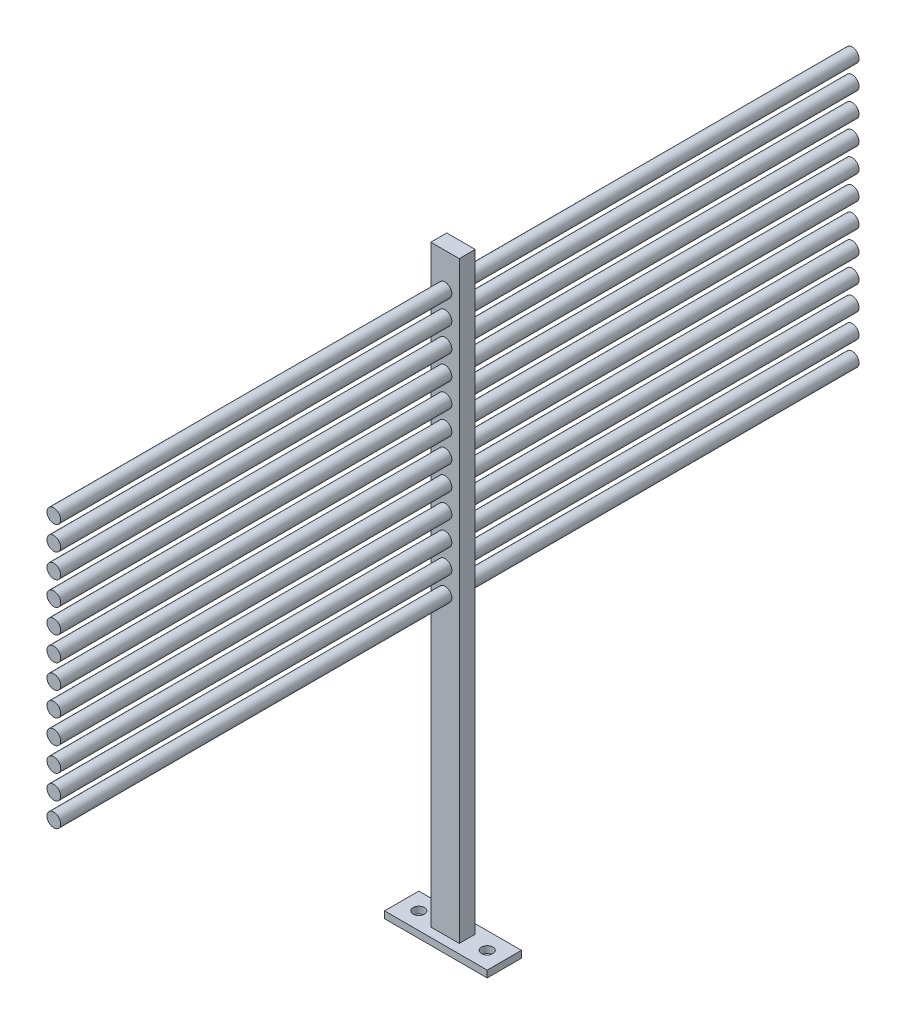
SolidWorks part; units mm, degrees
material "Q235"
ref_plane "Front Plane" through (0, 0, 0) normal (0, 0, 1) x (1, 0, 0)
ref_plane "Top Plane" through (0, 0, 0) normal (0, 1, 0) x (1, 0, 0)
ref_plane "Right Plane" through (0, 0, 0) normal (1, 0, 0) x (0, 0, -1)
sketch "Sketch1" plane through (0, 0, 0) normal (0, 0, 1) x (1, 0, 0)
  line L1 (-12.5, 260) -> (12.5, 260)
  line L2 (-12.5, 260) -> (-12.5, -260)
  line L3 (-12.5, -260) -> (12.5, -260)
  line L4 (12.5, 260) -> (12.5, -260)
  line L5 (-12.5, 260) -> (12.5, -260) construction
  line L6 (-12.5, -260) -> (12.5, 260) construction
  point P0 (0, 0)
  dimension "D1" = 25
  dimension "D2" = 520
extrude "Boss-Extrude1" add sketch "Sketch1" along normal blind 14
sketch "Sketch3" plane through (0, 0, 14) normal (0, 0, 1) x (1, 0, 0)
  line L0 (12.5, 260) -> (-12.5, 260) construction
  line L1 (12.5, -260) -> (12.5, 260) construction
  circle A0 centre (0, 230) radius 6
  dimension "D1" = 12
  dimension "D2" = 30
  dimension "D3" = 12.5
extrude "Boss-Extrude2" add sketch "Sketch3" along normal mid plane 700 from offset 7 offset against normal yes
pattern_linear "LPattern1" count 12 spacing 21 along (0, -1, 0) of "Boss-Extrude2"
sketch "Sketch4" plane through (0, -260, 0) normal (0, -1, 0) x (1, 0, 0)
  line L0 (-12.5, 14) -> (12.5, 0) construction
  line L2 (-45, 22) -> (45, 22)
  line L3 (-45, 22) -> (-45, -8)
  line L4 (-45, -8) -> (45, -8)
  line L5 (45, 22) -> (45, -8)
  line L6 (-45, 22) -> (45, -8) construction
  line L7 (-45, -8) -> (45, 22) construction
  point P4 (0, 7)
  dimension "D1" = 90
  dimension "D2" = 30
extrude "Boss-Extrude3" add sketch "Sketch4" along normal blind 6
sketch "Sketch5" plane through (0, 260, 0) normal (0, 1, 0) x (1, 0, 0)
  line L4 (-45, -22) -> (45, -22)
  line L5 (45, -22) -> (45, 8)
  line L6 (45, 8) -> (-45, 8)
  line L7 (-45, 8) -> (-45, -22)
  line L8 (-45, -22) -> (45, -22)
  line L9 (45, -22) -> (45, 8)
  line L10 (45, 8) -> (-45, 8)
  line L11 (-45, 8) -> (-45, -22)
  dimension "D1" = 0
extrude "Boss-Extrude4" [suppressed] add sketch "Sketch5" along normal blind 3
sketch "Sketch6" plane through (0, 0, 14) normal (0, 0, 1) x (1, 0, 0)
  line L0 (12.5, -260) -> (12.5, 260) construction
  circle A0 centre (0, 13.7774) radius 6
  dimension "D2" = 12
  dimension "D3" = 12.5
extrude "Cut-Extrude1" [suppressed] cut sketch "Sketch6" against normal through all
hole_wizard "M8 Clearance Hole1" positions "Sketch9" profile "Sketch10" hole size "M8" standard "GB"
sketch "Sketch9" plane through (0, -260, 0) normal (0, 1, 0) x (1, 0, 0)
  line L0 (0, 8) -> (0, 2.2866) construction
  line L1 (-45, 8) -> (45, 8) construction
  line L3 (-45, -7) -> (-30, -7) construction
  line L4 (-45, -22) -> (-45, 8) construction
  point P0 (-30, -7)
  point P2 (30, -7)
  dimension "D1" = 60
sketch "Sketch10" plane through (-30, -260, 7) normal (1, 0, 0) x (0, 0, 1)
  line L0 (0, 0) -> (0, 23.0043)
  line L1 (0, 23.0043) -> (5, 20)
  line L2 (5, 20) -> (5, 0)
  line L5 (5, 0) -> (0, 0)
  line L10 (0, 23.0043) -> (-5, 20) construction
  line L11 (0, -6.35) -> (0, 107.95) construction
  dimension "孔直径" = 10
  dimension "孔深度" = 20
  dimension "导头角度" = 118
